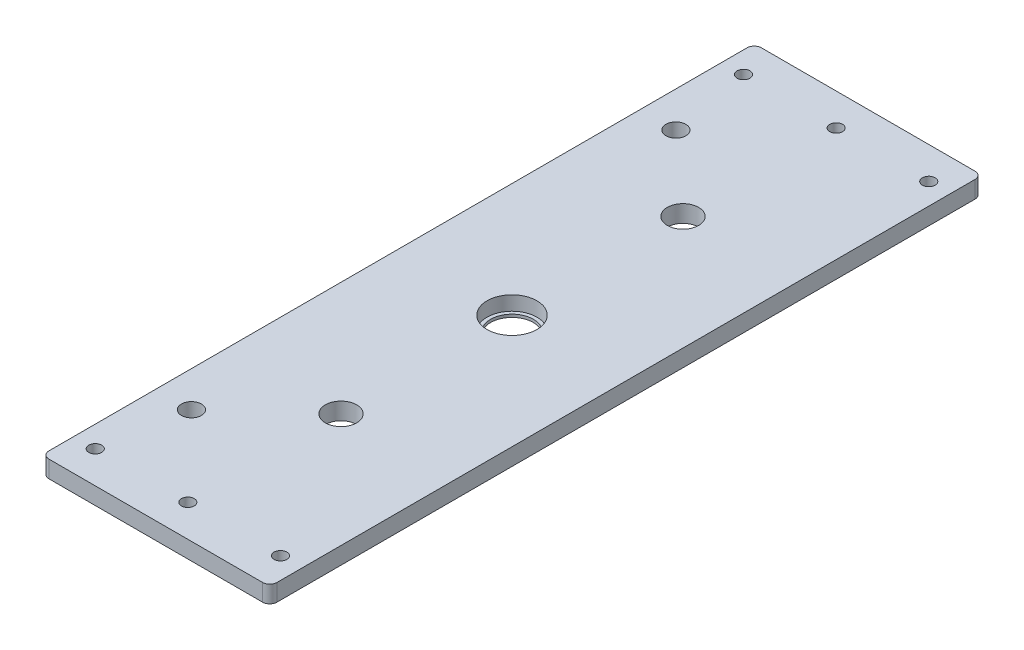
SolidWorks part; units mm, degrees
ref_plane "Front Plane" through (0, 0, 0) normal (0, 0, 1) x (1, 0, 0)
ref_plane "Top Plane" through (0, 0, 0) normal (0, 1, 0) x (1, 0, 0)
ref_plane "Right Plane" through (0, 0, 0) normal (1, 0, 0) x (0, 0, -1)
sketch "Sketch1" plane through (0, 0, 0) normal (0, 1, 0) x (1, 0, 0)
  line L1 (-80, -250) -> (80, -250)
  line L2 (-80, -250) -> (-80, 250)
  line L3 (-80, 250) -> (80, 250)
  line L4 (80, -250) -> (80, 250)
  line L5 (-80, -250) -> (80, 250) construction
  line L6 (-80, 250) -> (80, -250) construction
  point P0 (0, 0)
  dimension "D1" = 500
  dimension "D2" = 160
extrude "Boss-Extrude1" add sketch "Sketch1" along normal blind 12
sketch "Sketch2" plane through (0, 12, 0) normal (0, 1, 0) x (1, 0, 0)
  line L0 (0, -120) -> (0, 0) construction
  line L1 (0, 0) -> (-148.7179, 0) construction
  line L2 (80, 250) -> (-80, 250) construction
  circle A0 centre (0, 0) radius 15
  circle A2 centre (0, -120) radius 11
  circle A3 centre (0, 120) radius 11
  dimension "D1" = 30
  dimension "D2" = 130
  dimension "D3" = 22
extrude "Cut-Extrude1" cut sketch "Sketch2" against normal blind 12
sketch "Sketch3" plane through (0, 12, 0) normal (0, 1, 0) x (1, 0, 0)
  circle A0 centre (0, 0) radius 17.5
  dimension "D1" = 35
extrude "Cut-Extrude2" cut sketch "Sketch3" against normal blind 10
hole_wizard "Ø9.0 (9) Diameter Hole1" positions "Sketch5" profile "Sketch6" hole size "Ø9.0" standard "GB"
sketch "Sketch5" plane through (0, 12, 0) normal (0, 1, 0) x (1, 0, 0)
  line L2 (0, 0) -> (0, 227.5) construction
  line L3 (0, 227.5) -> (-65, 227.5) construction
  line L6 (65, 227.5) -> (0, 227.5) construction
  line L8 (80, 250) -> (-80, 250) construction
  line L9 (0, 0) -> (139.4616, 0) construction
  line L11 (65, -227.5) -> (0, -227.5) construction
  line L12 (0, -227.5) -> (-65, -227.5) construction
  line L13 (-130, 227.5) -> (-65, 227.5) construction
  line L18 (130, 227.5) -> (65, 227.5) construction
  point P0 (-65, 227.5)
  point P2 (0, 227.5)
  point P4 (65, 227.5)
  point P33 (-65, -227.5)
  point P36 (0, -227.5)
  point P39 (65, -227.5)
  dimension "D1" = 22.5
  dimension "D2" = 65
sketch "Sketch6" plane through (-65, 12, -227.5) normal (1, 0, 0) x (0, 0, 1)
  line L0 (0, 0) -> (0, 15.7039)
  line L1 (0, 15.7039) -> (4.5, 13)
  line L2 (4.5, 13) -> (4.5, 0)
  line L5 (4.5, 0) -> (0, 0)
  line L10 (0, 15.7039) -> (-4.5, 13) construction
  line L11 (0, -6.35) -> (0, 107.95) construction
  dimension "孔直径" = 9
  dimension "孔深度" = 13
  dimension "导头角度" = 118
fillet "Fillet1" radius 5 4 edges at (-80, 6, 250) (-80, 6, -250) (80, 6, -250) (80, 6, 250)
sketch "Sketch7" plane through (0, 0, 0) normal (0, -1, 0) x (1, 0, 0)
  line L0 (0, 0) -> (94.8932, 0) construction
  line L1 (-75, 250) -> (75, 250) construction
  line L3 (-80, -245) -> (-80, 245) construction
  circle A0 centre (-55, 170) radius 7
  circle A2 centre (-55, -170) radius 7
  dimension "D1" = 14
  dimension "D2" = 80
  dimension "D3" = 25
extrude "Cut-Extrude3" cut sketch "Sketch7" against normal through all
